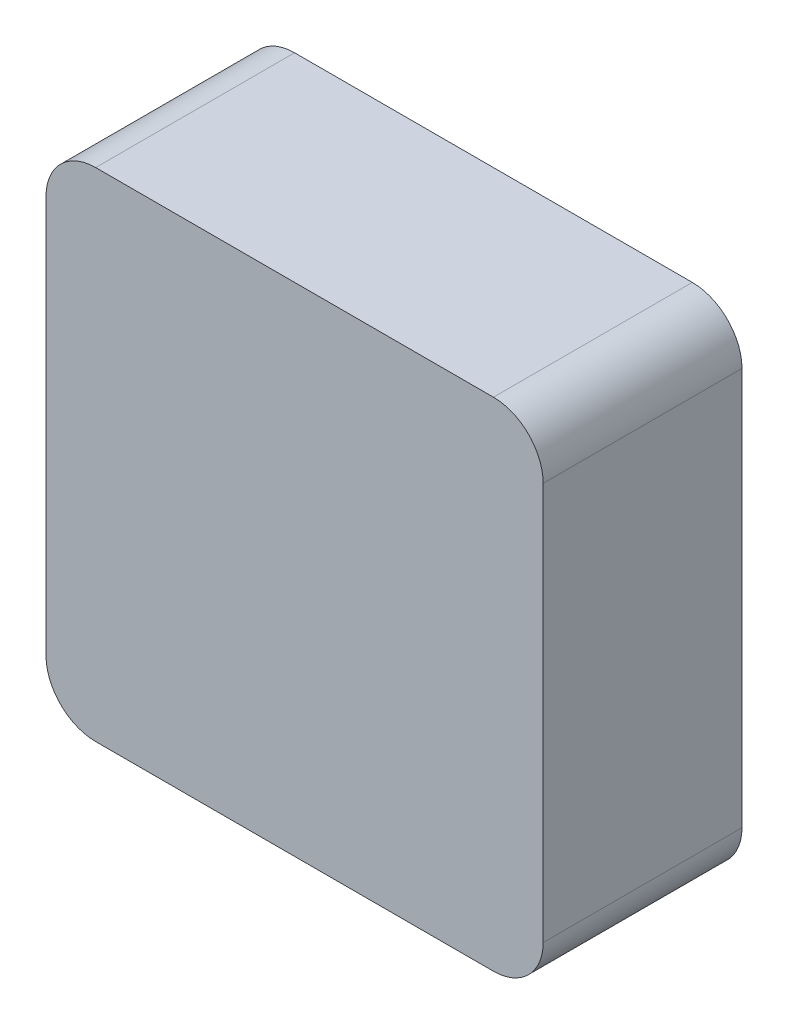
from build123d import *

# Parameters (mm, degrees)
SKETCH_1_W          = 100
SKETCH_1_H          = 100
EXTRUDE_1_DEPTH     = 40
SKETCH_2_R          = 37.5
CUT_EXTRUDE_1_DEPTH = 30
FILLET_1_R          = 10


with BuildPart() as part:
    # 草图1 → 凸台-拉伸1 (new body)
    with BuildSketch(Plane.XY):
        Rectangle(SKETCH_1_W, SKETCH_1_H)
    extrude(amount=EXTRUDE_1_DEPTH)

    # 草图2 → 切除-拉伸1 (cut)
    with BuildSketch(Plane(origin=(0, 0, 0), x_dir=(-1, 0, 0), z_dir=(0, 0, -1))):
        Circle(SKETCH_2_R)
    extrude(amount=-CUT_EXTRUDE_1_DEPTH, mode=Mode.SUBTRACT)

    # 圆角1
    fillet_1_edges = [part.edges().sort_by_distance(p)[0] for p in [
        (-50, -50, 20),
        (-50, 50, 20),
        (50, 50, 20),
        (50, -50, 20),
    ]]
    fillet(fillet_1_edges, radius=FILLET_1_R)


solid = part.part
